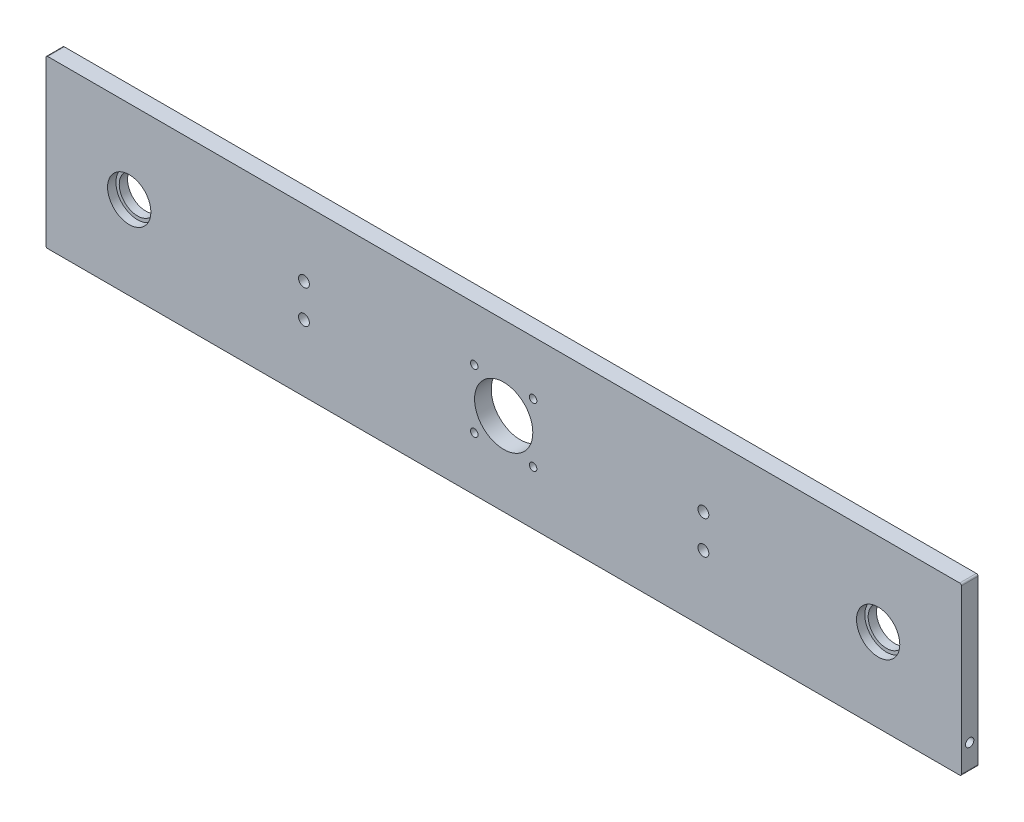
from build123d import *

# Parameters (mm, degrees)
SKETCH1_W           = 550
SKETCH1_H           = 100
BOSS_EXTRUDE1_DEPTH = 10
SKETCH3_R           = 13
CUT_EXTRUDE2_DEPTH  = 5
SKETCH4_R           = 11
CUT_EXTRUDE3_DEPTH  = 280.55321497
SKETCH5_R           = 17.5
CUT_EXTRUDE4_DEPTH  = 280.687325419
SKETCH6_R           = 2.25
CUT_EXTRUDE5_DEPTH  = 280.687325419
SKETCH7_R           = 3.25
CUT_EXTRUDE6_DEPTH  = 280.687325419
FILLET1_R           = 1


with BuildPart() as part:
    # Sketch1 → Boss-Extrude1 (new body)
    with BuildSketch(Plane.XY):
        Rectangle(SKETCH1_W, SKETCH1_H)
    extrude(amount=BOSS_EXTRUDE1_DEPTH)

    # Sketch3 → Cut-Extrude2 (cut)
    with BuildSketch(Plane.XY.offset(10)):
        with Locations((225, 0)):
            Circle(SKETCH3_R)
        with Locations(Location((-225, 0, 0), (0, 0, 180))):
            Circle(SKETCH3_R)
    extrude(amount=-CUT_EXTRUDE2_DEPTH, mode=Mode.SUBTRACT)

    # Sketch4 → Cut-Extrude3 (cut, through all)
    with BuildSketch(Plane.XY.offset(5)):
        with Locations((225, 0)):
            Circle(SKETCH4_R)
        with Locations(Location((-225, 0, 0), (0, 0, 180))):
            Circle(SKETCH4_R)
    extrude(amount=-CUT_EXTRUDE3_DEPTH, mode=Mode.SUBTRACT)

    # Sketch5 → Cut-Extrude4 (cut, through all)
    with BuildSketch(Plane.XY.offset(10)):
        Circle(SKETCH5_R)
    extrude(amount=-CUT_EXTRUDE4_DEPTH, mode=Mode.SUBTRACT)

    # Sketch6 → Cut-Extrude5 (cut, through all)
    with BuildSketch(Plane.XY.offset(10)):
        with Locations((-17.67766953, 17.67766953)):
            Circle(SKETCH6_R)
        with Locations((17.67766953, 17.67766953)):
            Circle(SKETCH6_R)
        with Locations((17.67766953, -17.67766953)):
            Circle(SKETCH6_R)
        with Locations((-17.67766953, -17.67766953)):
            Circle(SKETCH6_R)
    extrude(amount=-CUT_EXTRUDE5_DEPTH, mode=Mode.SUBTRACT)

    # Sketch7 → Cut-Extrude6 (cut, through all)
    with BuildSketch(Plane.XY.offset(10)):
        with Locations((-120, -10)):
            Circle(SKETCH7_R)
        with Locations((120, -10)):
            Circle(SKETCH7_R)
        with Locations((120, 10)):
            Circle(SKETCH7_R)
        with Locations((-120, 10)):
            Circle(SKETCH7_R)
    extrude(amount=-CUT_EXTRUDE6_DEPTH, mode=Mode.SUBTRACT)

    # Fillet1
    fillet1_edges = [part.edges().sort_by_distance(p)[0] for p in [
        (-275, 50, 5),
        (275, 50, 5),
        (275, -50, 5),
        (-275, -50, 5),
    ]]
    fillet(fillet1_edges, radius=FILLET1_R)

    # Sketch9 → M6 Tapped Hole1 (revolve, cut)
    with BuildSketch(Plane(origin=(-275, -35, 5), x_dir=(0, 0, 1), z_dir=(0, 1, 0))):
        Polygon((0, 0), (0, 19.502151548), (2.5, 18), (2.5, 0), align=None)
    m6_tapped_hole1 = revolve(axis=Axis((-281.35, -35, 5), (1, 0, 0)), mode=Mode.SUBTRACT)

    # Mirror1: M6 Tapped Hole1 across plane
    add(m6_tapped_hole1.mirror(Plane(origin=(0, 0, 0), x_dir=(0, 0, 1), z_dir=(1, 0, 0))), mode=Mode.SUBTRACT)


solid = part.part
